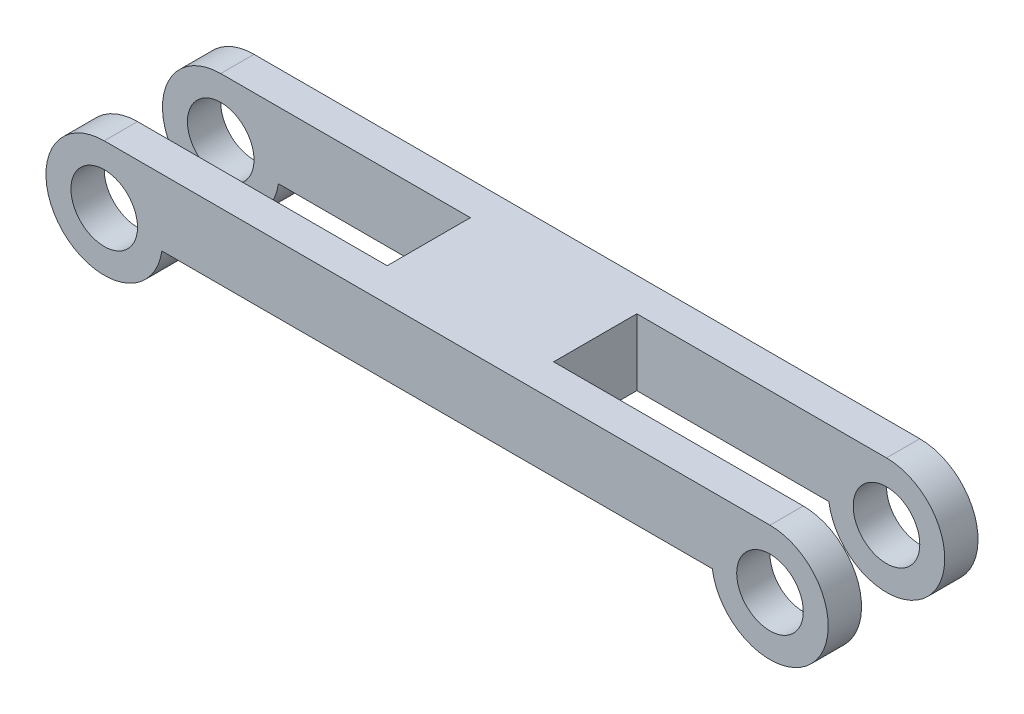
SolidWorks part; units mm, degrees
ref_plane "Front Plane" through (0, 0, 0) normal (0, 0, 1) x (1, 0, 0)
ref_plane "Top Plane" through (0, 0, 0) normal (0, 1, 0) x (1, 0, 0)
ref_plane "Right Plane" through (0, 0, 0) normal (1, 0, 0) x (0, 0, -1)
other "Configuration Table"
sketch "Sketch1" plane through (0, 0, 0) normal (0, 0, 1) x (1, 0, 0)
  line L0 (-20, 3.5) -> (20, 3.5)
  line L1 (-16.5359, -0.5) -> (16.5359, -0.5)
  circle A0 centre (20, 0) radius 2
  circle A1 centre (-20, 0) radius 2
  arc A2 (-20, 3.5) -> (-16.5359, -0.5) centre (-20, 0) ccw
  arc A3 (16.5359, -0.5) -> (20, 3.5) centre (20, 0) ccw
  point P2 (0, 3.5)
  dimension "D1" = 4
  dimension "D2" = 3.5
  dimension "D3" = 16.5359
  dimension "D4" = 20
extrude "Boss-Extrude1" add sketch "Sketch1" along normal blind 9
sketch "Sketch2" plane through (0, 3.5, 0) normal (0, 1, 0) x (1, 0, 0)
  line L0 (-23.5, 0) -> (-23.5, -9) construction
  line L1 (-42, -2) -> (-5, -2)
  line L2 (-42, -2) -> (-42, -7)
  line L3 (-42, -7) -> (-5, -7)
  line L4 (-5, -2) -> (-5, -7)
  line L5 (-23.5, -7) -> (-23.5, -2) construction
  line L6 (-42, -4.5) -> (-5, -4.5) construction
  point P0 (-23.5, -4.5)
  dimension "D1" = 5
  dimension "D2" = 5
extrude "Cut-Extrude1" cut sketch "Sketch2" against normal blind 9
mirror "Mirror1" about plane through (0, 0, 0) normal (1, 0, 0) of "Cut-Extrude1"
